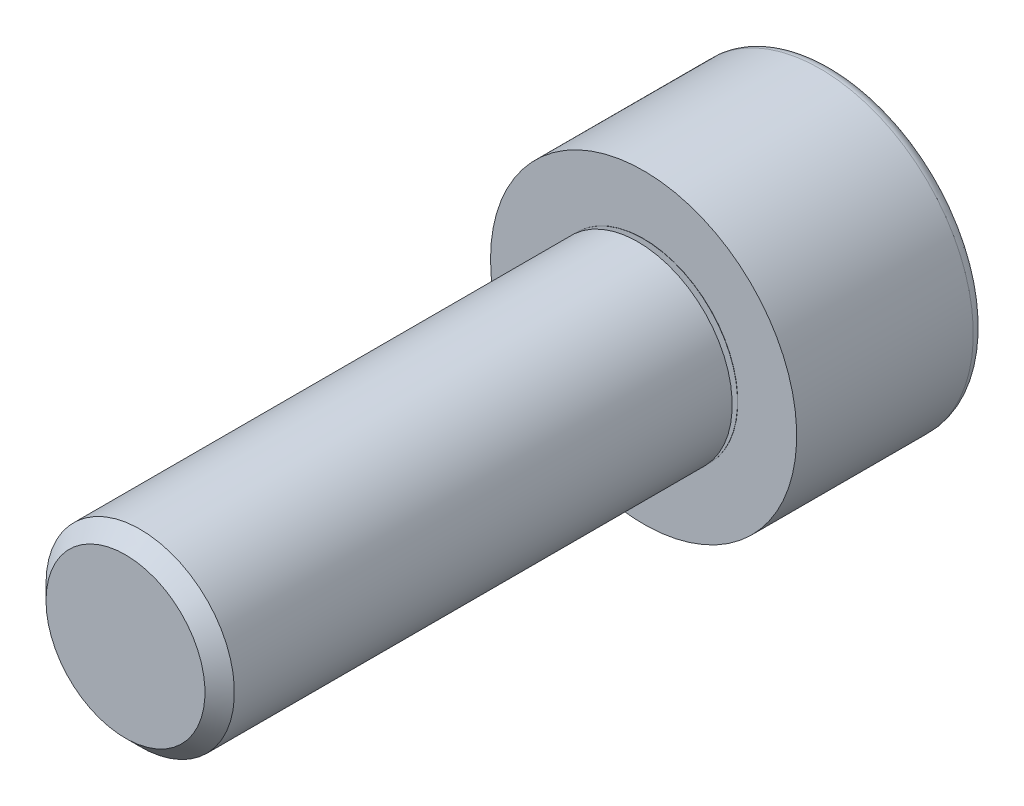
from build123d import *

# Parameters (mm, degrees)
CUT_EXTRUDE1_DEPTH = 3


with BuildPart() as part:
    # Logo3_bib1 → Revolve1 (revolve)
    with BuildSketch(Plane(origin=(0, 0, 0), x_dir=(-1, 0, 0), z_dir=(0, -1, 0))):
        with BuildLine():
            Line((0, -22), (0, 8))
            Line((0, 8), (6, 8))
            ThreePointArc((6, 8), (6.353553391, 7.853553391), (6.5, 7.5))
            Line((6.5, 7.5), (6.5, 0))
            Line((6.5, 0), (4, 0))
            Line((4, 0), (4, -0.01))
            Line((4, -0.01), (3.488425636, -0.01))
            ThreePointArc((3.488425636, -0.01), (3.468729481, -0.026527036), (3.481585234, -0.048793852))
            Line((3.481585234, -0.048793852), (4, -0.237481396))
            Line((4, -0.237481396), (4, -21.375))
            Line((4, -21.375), (3.375, -22))
            Line((3.375, -22), (0, -22))
        make_face()
    revolve(axis=Axis((0, 0, -10.585154653), (0, 0, 1)))

    # Logo3_bib2 → Cut-Extrude1 (cut)
    with BuildSketch(Plane(origin=(0, 0, -8), x_dir=(1, 0, 0), z_dir=(0, 0, -1))):
        Polygon((3.464101615, 0), (1.732050808, 3), (-1.732050808, 3), (-3.464101615, 0), (-1.732050808, -3), (1.732050808, -3), align=None)
    extrude(amount=-CUT_EXTRUDE1_DEPTH, mode=Mode.SUBTRACT)


solid = part.part
